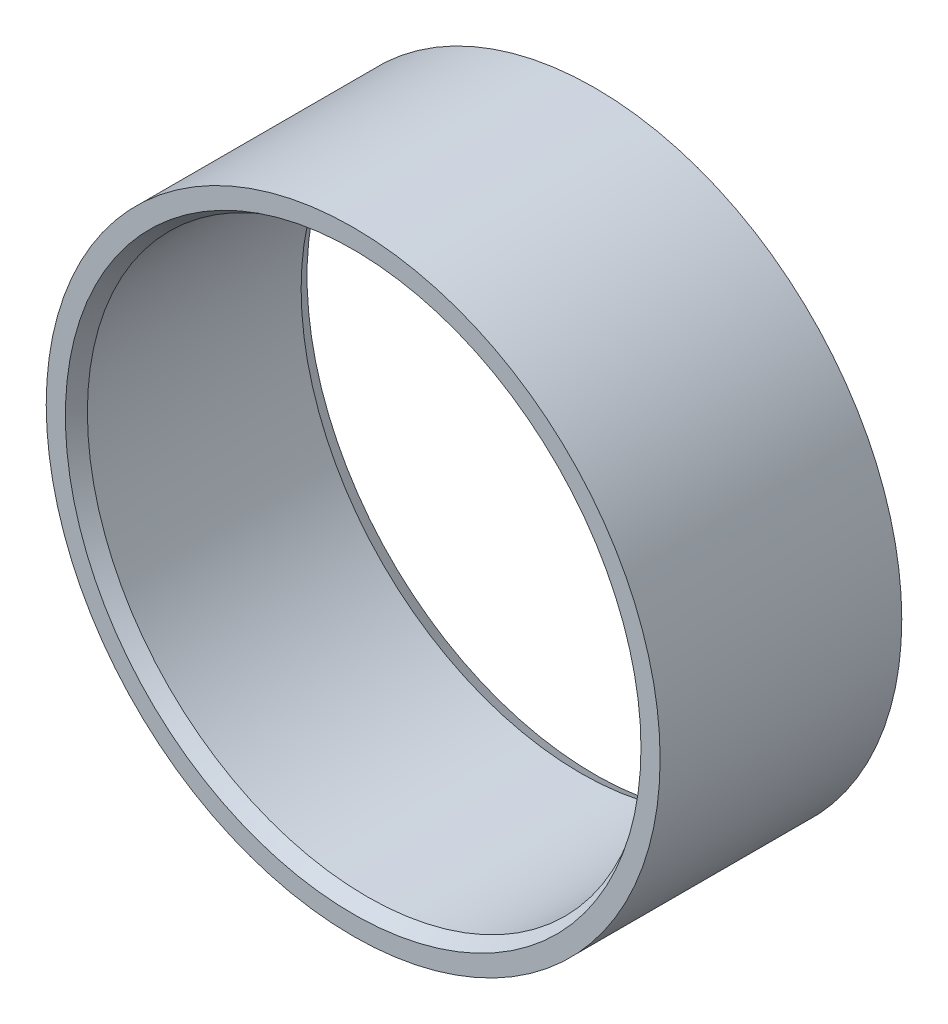
from build123d import *

# Parameters (mm, degrees)
SKETCH_1_R      = 11
SKETCH_1_R_2    = 10.025
EXTRUDE_1_DEPTH = 8.66
CHAMFER_1_SIZE  = 0.5
CHAMFER_1_SIZE2 = 0.288675135


with BuildPart() as part:
    # 草图1 → 凸台-拉伸1 (new body)
    with BuildSketch(Plane.XY):
        Circle(SKETCH_1_R)
        Circle(SKETCH_1_R_2, mode=Mode.SUBTRACT)
    extrude(amount=EXTRUDE_1_DEPTH)

    # 倒角1
    chamfer_1_edges = [part.edges().sort_by_distance(p)[0] for p in [
        (-10.025, 0, 0),
        (-10.025, 0, 8.66),
    ]]
    chamfer_1_side = [part.faces().sort_by_distance(p)[0] for p in [
        (-10.025, 0, 4.33),
    ]]
    chamfer(chamfer_1_edges, length=CHAMFER_1_SIZE, length2=CHAMFER_1_SIZE2, reference=chamfer_1_side[0])


solid = part.part
